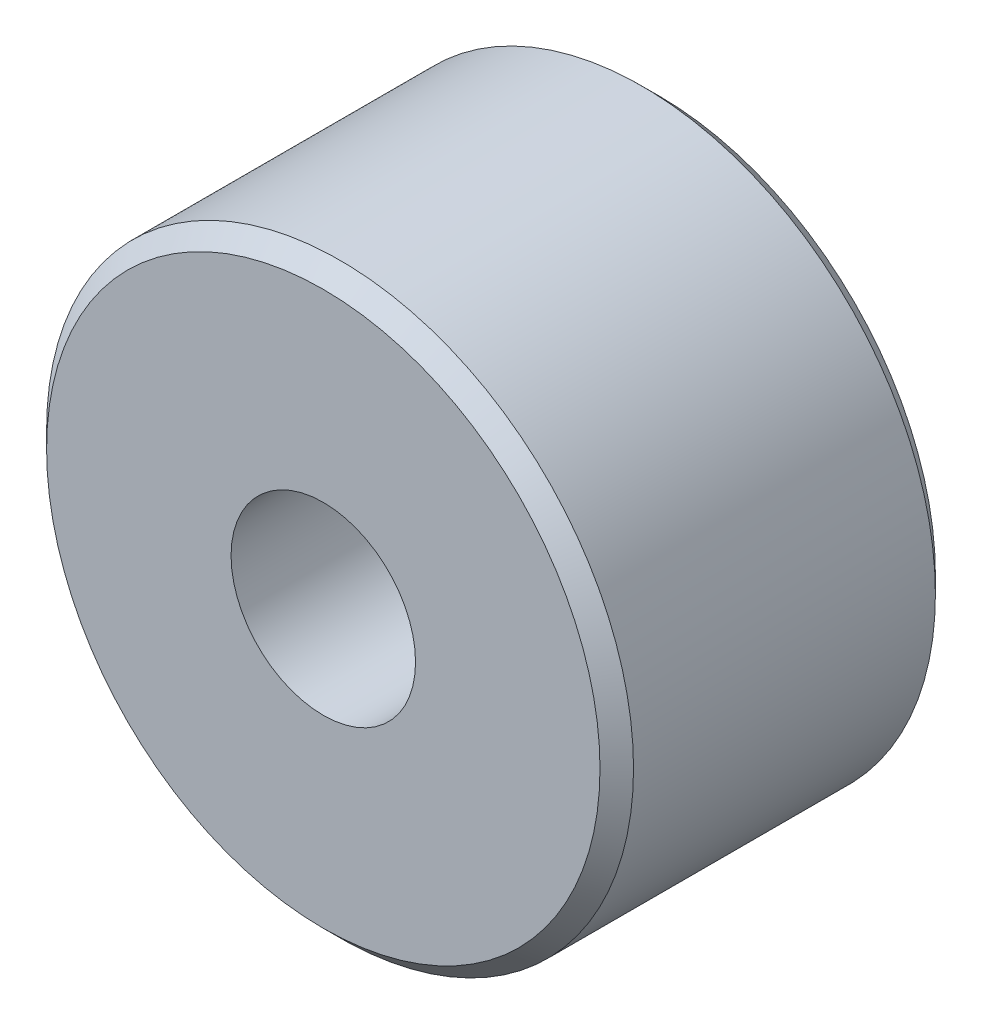
from build123d import *

# Parameters (mm, degrees)
SKETCH1_R           = 8.75
SKETCH1_R_2         = 2.75
BOSS_EXTRUDE1_DEPTH = 10
SKETCH2_R           = 5
CUT_EXTRUDE1_DEPTH  = 5.5
CHAMFER1_SIZE       = 0.5


with BuildPart() as part:
    # Sketch1 → Boss-Extrude1 (new body)
    with BuildSketch(Plane.XY):
        Circle(SKETCH1_R)
        Circle(SKETCH1_R_2, mode=Mode.SUBTRACT)
    extrude(amount=BOSS_EXTRUDE1_DEPTH)

    # Sketch2 → Cut-Extrude1 (cut)
    with BuildSketch(Plane(origin=(0, 0, 0), x_dir=(-1, 0, 0), z_dir=(0, 0, -1))):
        Circle(SKETCH2_R)
    extrude(amount=-CUT_EXTRUDE1_DEPTH, mode=Mode.SUBTRACT)

    # Chamfer1
    chamfer1_edges = [part.edges().sort_by_distance(p)[0] for p in [
        (-8.75, 0, 0),
        (-8.75, 0, 10),
    ]]
    chamfer(chamfer1_edges, length=CHAMFER1_SIZE)


solid = part.part
